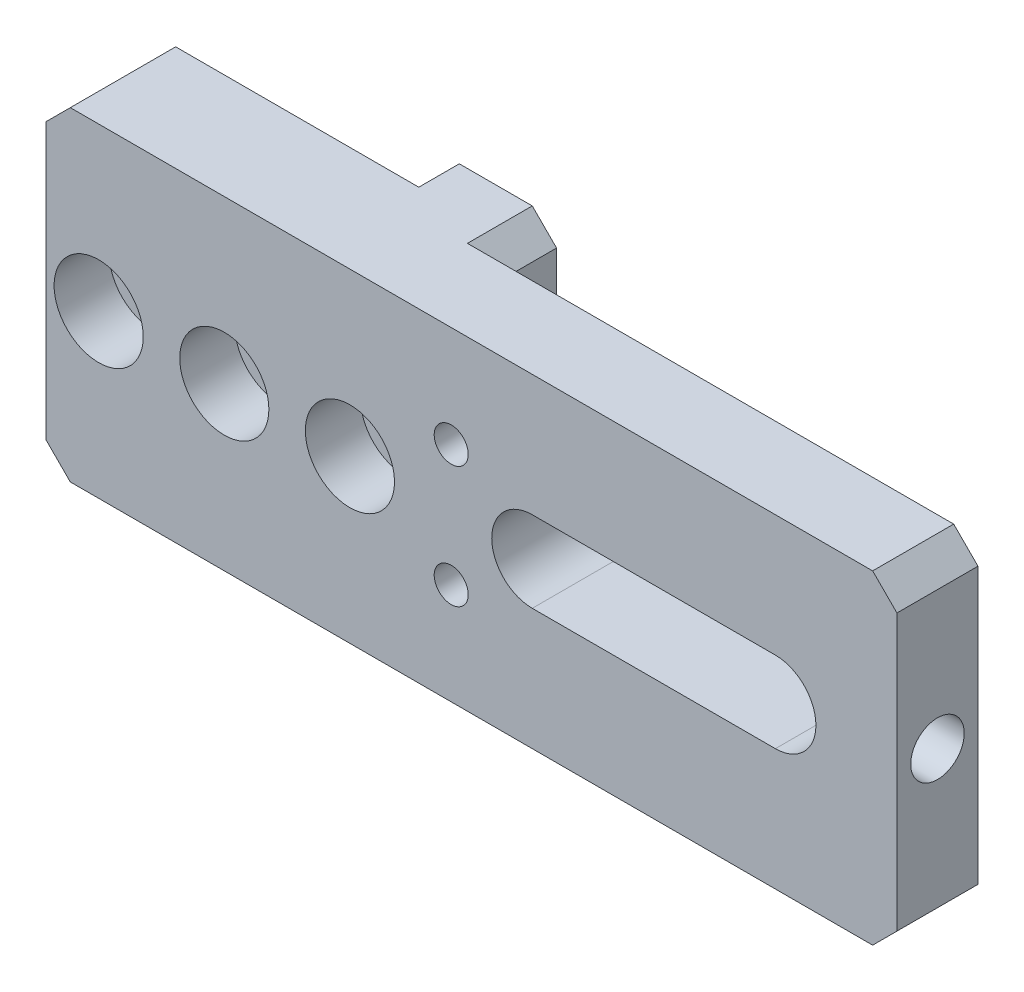
from build123d import *

# Parameters (mm, degrees)
SKETCH_1_W                = 105
SKETCH_1_H                = 40
EXTRUDE_1_DEPTH           = 18
SKETCH_2_W                = 30
SKETCH_2_H                = 40
CUT_EXTRUDE_1_DEPTH       = 5
SKETCH_3_W                = 60
SKETCH_3_H                = 40
CUT_EXTRUDE_2_DEPTH       = 8
HOLE_WIZARD_1_D           = 6.6
HOLE_WIZARD_1_CBORE_D     = 11
HOLE_WIZARD_1_CBORE_DEPTH = 6.8
SKETCH_6_R                = 5
CUT_EXTRUDE_3_DEPTH       = 2
CHAMFER_1_SIZE            = 3
CUT_EXTRUDE_4_DEPTH       = 59.993643725
HOLE_WIZARD_M6_1_REACH    = 110.393
HOLE_WIZARD_M6_1_BORE_R   = 3.3
HOLE_WIZARD_M5_1_D        = 4.2


with BuildPart() as part:
    # 草图1 → 凸台-拉伸1 (new body)
    with BuildSketch(Plane.XY):
        Rectangle(SKETCH_1_W, SKETCH_1_H)
    extrude(amount=EXTRUDE_1_DEPTH)

    # 草图2 → 切除-拉伸1 (cut)
    with BuildSketch(Plane(origin=(0, 0, 0), x_dir=(-1, 0, 0), z_dir=(0, 0, -1))):
        with Locations((37.5, 0)):
            Rectangle(SKETCH_2_W, SKETCH_2_H)
    extrude(amount=-CUT_EXTRUDE_1_DEPTH, mode=Mode.SUBTRACT)

    # 草图3 → 切除-拉伸2 (cut)
    with BuildSketch(Plane(origin=(0, 0, 0), x_dir=(-1, 0, 0), z_dir=(0, 0, -1))):
        with Locations((-22.5, 0)):
            Rectangle(SKETCH_3_W, SKETCH_3_H)
    extrude(amount=-CUT_EXTRUDE_2_DEPTH, mode=Mode.SUBTRACT)

    # 打孔尺寸(%根据)内六角圆柱头螺钉的类型1 (through all)
    with Locations(Plane.XY.offset(18)):
        with Locations((-46, 0), (-30.5, 0), (-15, 0)):
            CounterBoreHole(HOLE_WIZARD_1_D / 2, HOLE_WIZARD_1_CBORE_D / 2, HOLE_WIZARD_1_CBORE_DEPTH)

    # 草图6 → 切除-拉伸3 (cut)
    with BuildSketch(Plane(origin=(0, 0, 0), x_dir=(-1, 0, 0), z_dir=(0, 0, -1))):
        with Locations((15, 0)):
            Circle(SKETCH_6_R)
    extrude(amount=-CUT_EXTRUDE_3_DEPTH, mode=Mode.SUBTRACT)

    # 倒角1
    chamfer_1_edges = [part.edges().sort_by_distance(p)[0] for p in [
        (-22.5, -20, 2.5),
        (-22.5, 20, 2.5),
        (-7.5, 20, 4),
        (-7.5, -20, 4),
        (52.5, -20, 13),
        (-52.5, -20, 11.5),
        (-52.5, 20, 11.5),
        (52.5, 20, 13),
    ]]
    chamfer(chamfer_1_edges, length=CHAMFER_1_SIZE)

    # 草图7 → 切除-拉伸4 (cut, through all)
    with BuildSketch(Plane.XY.offset(18)):
        with BuildLine():
            Line((7.5, 5), (37.5, 5))
            ThreePointArc((37.5, 5), (42.5, 0), (37.5, -5))
            Line((37.5, -5), (7.5, -5))
            ThreePointArc((7.5, -5), (2.5, 0), (7.5, 5))
        make_face()
    extrude(amount=-CUT_EXTRUDE_4_DEPTH, mode=Mode.SUBTRACT)

    # M6 间隙孔1 bore → M6 间隙孔1 (cut, up to next)
    with BuildSketch(Plane(origin=(52.5, 0, 0), x_dir=(0, 0, -1), z_dir=(1, 0, 0)), mode=Mode.PRIVATE) as hole_wizard_m6_1_sk1:
        with Locations((-13, 0)):
            Circle(HOLE_WIZARD_M6_1_BORE_R)
    hole_wizard_m6_1_tool1 = extrude(hole_wizard_m6_1_sk1.sketch, amount=-HOLE_WIZARD_M6_1_REACH, mode=Mode.PRIVATE) & part.part
    add(hole_wizard_m6_1_tool1.solids().sort_by_distance((52.5, 0, 13))[0], mode=Mode.SUBTRACT)

    # M5 螺纹孔1 (through all)
    with Locations(Plane.XY.offset(18)):
        with Locations((-2.5, 7.5), (-2.5, -7.5)):
            Hole(HOLE_WIZARD_M5_1_D / 2)


solid = part.part
